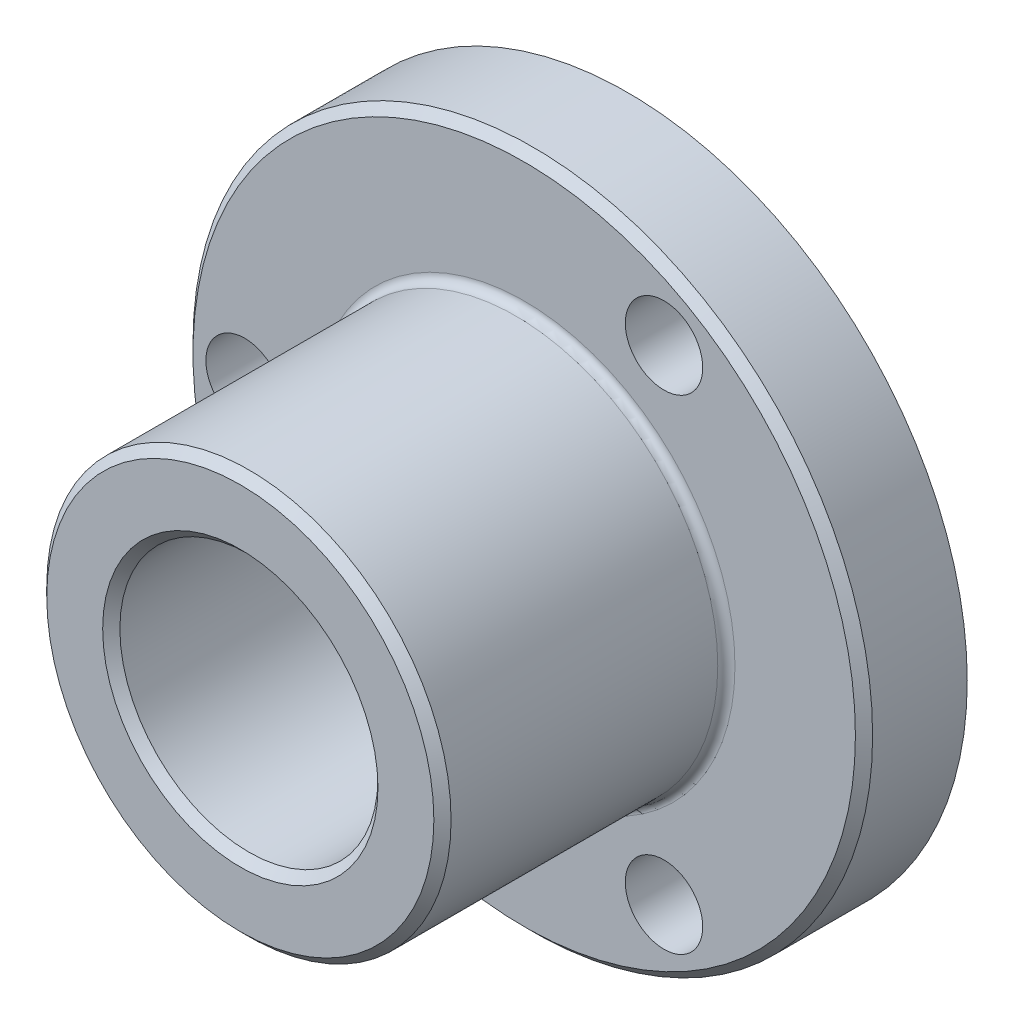
from build123d import *

# Parameters (mm, degrees)
SKETCH1_R           = 39.5
BOSS_EXTRUDE1_DEPTH = 12
SKETCH2_R           = 23.5
BOSS_EXTRUDE2_DEPTH = 33
SKETCH3_R           = 15
CUT_EXTRUDE1_DEPTH  = 35
SKETCH4_R           = 5.5
CUT_EXTRUDE2_DEPTH  = 3
SKETCH5_R           = 5.5
CUT_EXTRUDE3_DEPTH  = 7
CUT_EXTRUDE3_DRAFT  = 45
CHAMFER1_SIZE       = 1
SKETCH6_R           = 4.5
CUT_EXTRUDE4_DEPTH  = 21
FILLET1_R           = 1


with BuildPart() as part:
    # Sketch1 → Boss-Extrude1 (new body)
    with BuildSketch(Plane.XY):
        Circle(SKETCH1_R)
    extrude(amount=BOSS_EXTRUDE1_DEPTH)

    # Sketch2 → Boss-Extrude2 (add)
    with BuildSketch(Plane.XY.offset(12)):
        Circle(SKETCH2_R)
    extrude(amount=BOSS_EXTRUDE2_DEPTH)

    # Sketch3 → Cut-Extrude1 (cut)
    with BuildSketch(Plane.XY.offset(45)):
        Circle(SKETCH3_R)
    extrude(amount=-CUT_EXTRUDE1_DEPTH, mode=Mode.SUBTRACT)

    # Sketch4 → Cut-Extrude2 (cut)
    with BuildSketch(Plane.XY.offset(10)):
        Circle(SKETCH4_R)
    extrude(amount=-CUT_EXTRUDE2_DEPTH, mode=Mode.SUBTRACT)


with BuildPart() as cut_extrude3_tool:
    # Sketch5 → Cut-Extrude3 (with draft: the straight prism first)
    with BuildSketch(Plane.XY.offset(7)):
        Circle(SKETCH5_R)
    extrude(amount=-CUT_EXTRUDE3_DEPTH)
    # Cut-Extrude3: the draft: its side faces are tilted about the plane it starts from
    cut_extrude3_sides = [cut_extrude3_tool.faces().sort_by_distance(p)[0] for p in [
        (-5.5, 0, 3.5),
    ]]
    draft(cut_extrude3_sides, Plane.XY.offset(7), CUT_EXTRUDE3_DRAFT)


with BuildPart() as part_1:
    add(part.part)

    # Cut-Extrude3: cut by cut_extrude3_tool
    add(cut_extrude3_tool.part, mode=Mode.SUBTRACT)

    # Chamfer1
    chamfer1_edges = [part_1.edges().sort_by_distance(p)[0] for p in [
        (-15, 0, 45),
        (-39.5, 0, 12),
        (-23.5, 0, 45),
    ]]
    chamfer(chamfer1_edges, length=CHAMFER1_SIZE)

    # Sketch6 → Cut-Extrude4 (cut)
    with BuildSketch(Plane(origin=(0, 0, 0), x_dir=(-1, 0, 0), z_dir=(0, 0, -1))):
        with Locations((32.5, 0)):
            Circle(SKETCH6_R)
        with Locations((-16.25, -28.145825623)):
            Circle(SKETCH6_R)
        with Locations((-16.25, 28.145825623)):
            Circle(SKETCH6_R)
    extrude(amount=-CUT_EXTRUDE4_DEPTH, mode=Mode.SUBTRACT)

    # Fillet1
    fillet1_edges = [part_1.edges().sort_by_distance(p)[0] for p in [
        (-15, 0, 10),
        (-23.5, 0, 12),
    ]]
    fillet(fillet1_edges, radius=FILLET1_R)


solid = part_1.part
